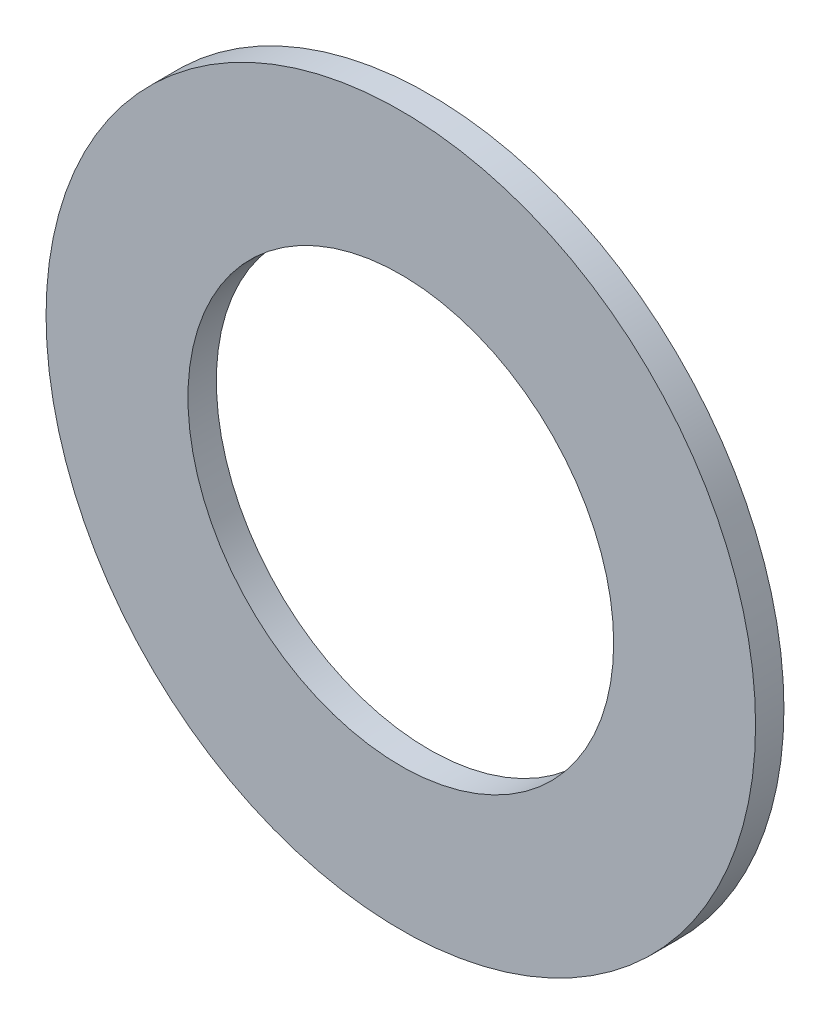
from build123d import *

# Parameters (mm, degrees)
SKETCH1_R           = 2.5
SKETCH1_R_2         = 1.5
BOSS_EXTRUDE1_DEPTH = 0.2


with BuildPart() as part:
    # Sketch1 → Boss-Extrude1 (new body)
    with BuildSketch(Plane.XY):
        Circle(SKETCH1_R)
        Circle(SKETCH1_R_2, mode=Mode.SUBTRACT)
    extrude(amount=BOSS_EXTRUDE1_DEPTH)


solid = part.part
